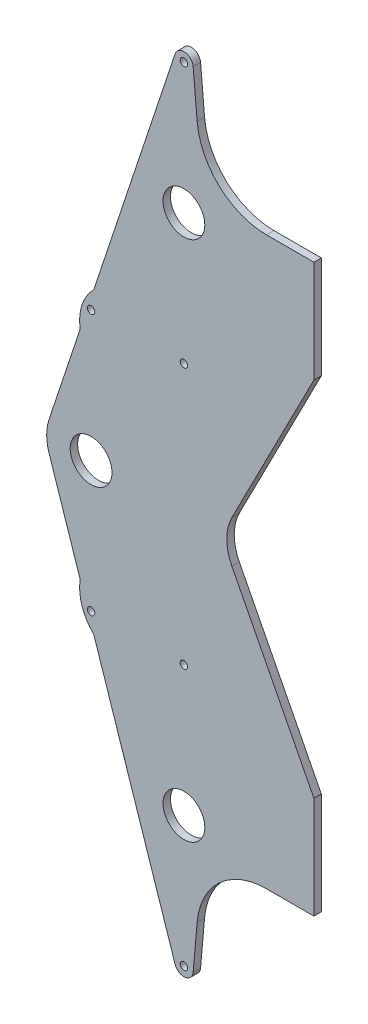
from build123d import *

# Parameters (mm, degrees)
SKETCH1_R           = 45
SKETCH1_R_2         = 3.5
SKETCH1_R_3         = 8
BOSS_EXTRUDE1_DEPTH = 16
BOSS_EXTRUDE2_START = -16
SKETCH4_R           = 3.5
BOSS_EXTRUDE2_DEPTH = 16


with BuildPart() as part:
    # Sketch1 → Boss-Extrude1 (new body)
    with BuildSketch(Plane.XY):
        with BuildLine():
            Line((-570.535490362, 31.513955821), (-503.404469767, 233.679569935))
            ThreePointArc((-503.404469767, 233.679569935), (-499.566128801, 281), (-474.336723785, 321.217323201))
            Line((-474.336723785, 321.217323201), (-298.980906816, 849.302791164))
            ThreePointArc((-298.980906816, 849.302791164), (-277.671917484, 862.864038658), (-260.076106038, 844.743114855))
            Line((-260.076106038, 844.743114855), (-251.518273259, 746.926638588))
            ThreePointArc((-251.518273259, 746.926638588), (-203.427599687, 649.408399478), (-102.089068545, 610))
            Line((-102.089068545, 610), (0, 610))
            Line((0, 610), (0, 390))
            Line((0, 390), (-176.599146277, 45.63166476))
            ThreePointArc((-176.599146277, 45.63166476), (-187.617399996, 0), (-176.599146277, -45.63166476))
            Line((-176.599146277, -45.63166476), (0, -390))
            Line((0, -390), (0, -610))
            Line((0, -610), (-102.089068545, -610))
            ThreePointArc((-102.089068545, -610), (-203.427599687, -649.408399478), (-251.518273259, -746.926638588))
            Line((-251.518273259, -746.926638588), (-260.076106038, -844.743114855))
            ThreePointArc((-260.076106038, -844.743114855), (-277.671917484, -862.864038658), (-298.980906816, -849.302791164))
            Line((-298.980906816, -849.302791164), (-474.336723785, -321.217323201))
            ThreePointArc((-474.336723785, -321.217323201), (-499.566128801, -281), (-503.404469767, -233.679569935))
            Line((-503.404469767, -233.679569935), (-570.535490362, -31.513955821))
            ThreePointArc((-570.535490362, -31.513955821), (-575.630956285, 0), (-570.535490362, 31.513955821))
        make_face()
        with Locations((-280, 562)):
            Circle(SKETCH1_R, mode=Mode.SUBTRACT)
        with Locations((-355, 582)):
            Circle(SKETCH1_R_2, mode=Mode.SUBTRACT)
        with Locations((-280, 281)):
            Circle(SKETCH1_R_3, mode=Mode.SUBTRACT)
        with Locations((-355, -582)):
            Circle(SKETCH1_R_2, mode=Mode.SUBTRACT)
        with Locations((-355, -542)):
            Circle(SKETCH1_R_2, mode=Mode.SUBTRACT)
        with Locations((-405, -20)):
            Circle(SKETCH1_R_2, mode=Mode.SUBTRACT)
        with Locations((-405, 20)):
            Circle(SKETCH1_R_2, mode=Mode.SUBTRACT)
        with Locations((-280, 843)):
            Circle(SKETCH1_R_3, mode=Mode.SUBTRACT)
        with Locations((-280, -843)):
            Circle(SKETCH1_R_3, mode=Mode.SUBTRACT)
        with Locations((-280, -281)):
            Circle(SKETCH1_R_3, mode=Mode.SUBTRACT)
        with Locations((-480, -281)):
            Circle(SKETCH1_R_3, mode=Mode.SUBTRACT)
        with Locations((-280, -562)):
            Circle(SKETCH1_R, mode=Mode.SUBTRACT)
        with Locations((-480, 0)):
            Circle(SKETCH1_R, mode=Mode.SUBTRACT)
        with Locations((-480, 281)):
            Circle(SKETCH1_R_3, mode=Mode.SUBTRACT)
        with Locations((-355, 542)):
            Circle(SKETCH1_R_2, mode=Mode.SUBTRACT)
    extrude(amount=BOSS_EXTRUDE1_DEPTH)

    # Sketch4 → Boss-Extrude2 (add)
    with BuildSketch(Plane.XY.offset(16).offset(BOSS_EXTRUDE2_START)):
        with Locations((-355, -542)):
            Circle(SKETCH4_R)
        with Locations((-355, -582)):
            Circle(SKETCH4_R)
        with Locations((-405, -20)):
            Circle(SKETCH4_R)
        with Locations((-405, 20)):
            Circle(SKETCH4_R)
        with Locations((-355, 542)):
            Circle(SKETCH4_R)
        with Locations((-355, 582)):
            Circle(SKETCH4_R)
    extrude(amount=BOSS_EXTRUDE2_DEPTH)


solid = part.part
